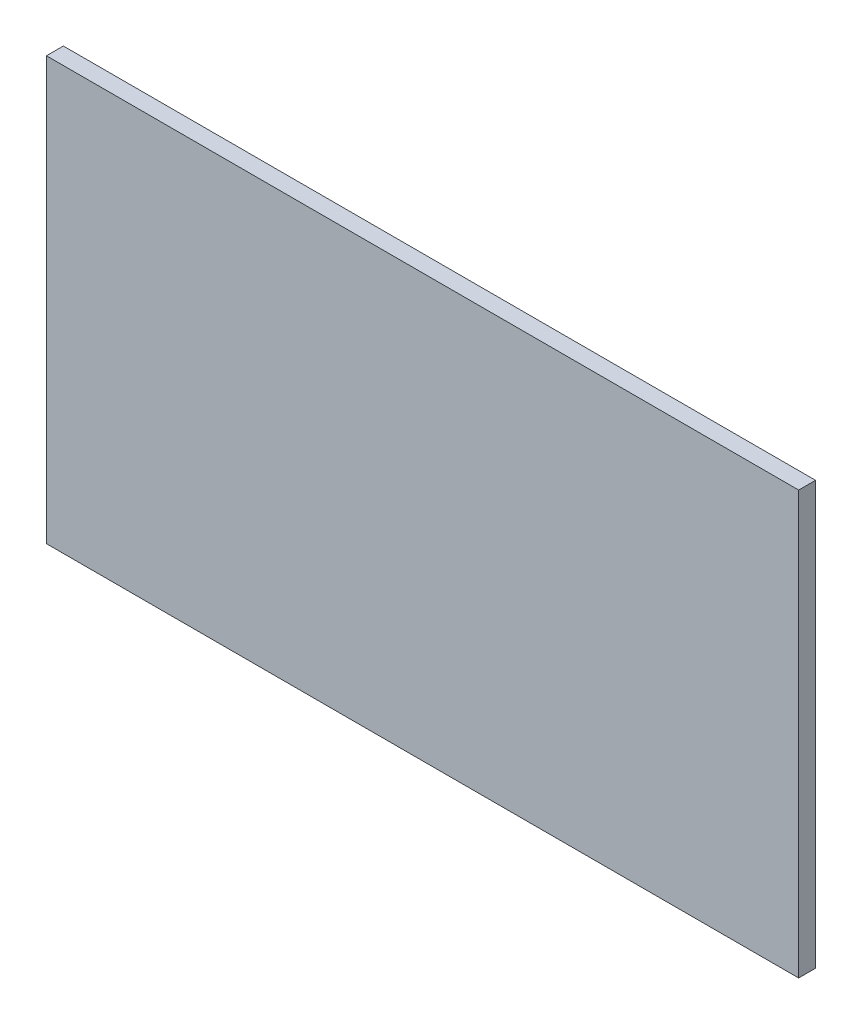
SolidWorks part; units mm, degrees
material "Q235B"
ref_plane "Front Plane" through (0, 0, 0) normal (0, 0, 1) x (1, 0, 0)
ref_plane "Top Plane" through (0, 0, 0) normal (0, 1, 0) x (1, 0, 0)
ref_plane "Right Plane" through (0, 0, 0) normal (1, 0, 0) x (0, 0, -1)
sketch "Sketch1" plane through (0, 0, 0) normal (0, 0, 1) x (1, 0, 0)
  line L2 (0, 0) -> (0, 1000)
  line L3 (0, 1000) -> (1780, 1000)
  line L4 (1780, 500) -> (1780, 1000)
  line L7 (0, 0) -> (1780, 0)
  line L8 (1780, 500) -> (1780, 0)
  dimension "D2" = 1000
  dimension "D4" = 1780
extrude "Boss-Extrude1" add sketch "Sketch1" along normal blind 40
